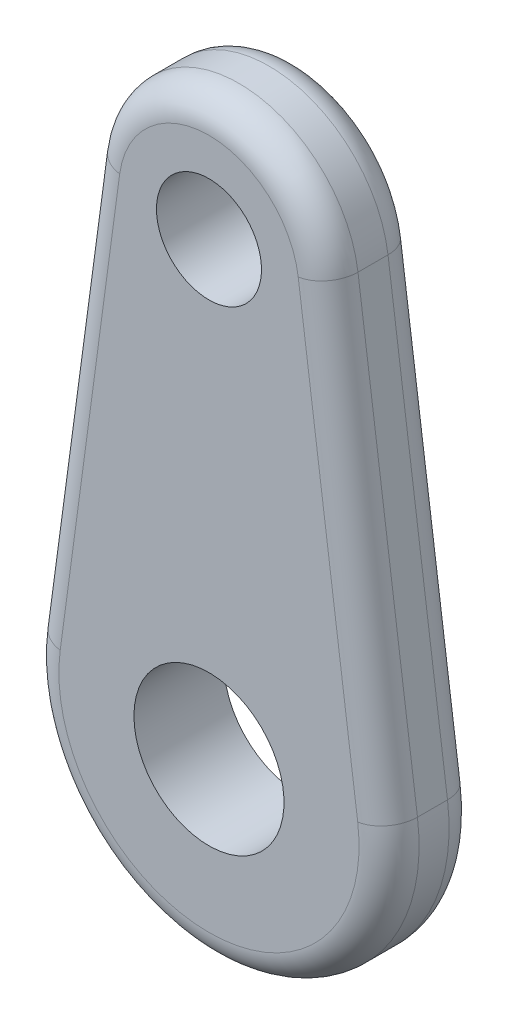
from build123d import *

# Parameters (mm, degrees)
BOSS_EXTRUDE1_DEPTH   = 30
M30_CLEARANCE_HOLE1_D = 35
M45_CLEARANCE_HOLE1_D = 50
FILLET1_R             = 10


with BuildPart() as part:
    # Sketch1 → Boss-Extrude1 (new body)
    with BuildSketch(Plane.XY.offset(30)):
        with BuildLine():
            Line((59.464274989, 8), (39.642849993, 155.333333333))
            ThreePointArc((39.642849993, 155.333333333), (0, 190), (-39.642849993, 155.333333333))
            Line((-39.642849993, 155.333333333), (-59.464274989, 8))
            ThreePointArc((-59.464274989, 8), (0, -60), (59.464274989, 8))
        make_face()
    extrude(amount=-BOSS_EXTRUDE1_DEPTH)

    # M30 Clearance Hole1 (through all)
    with Locations(Plane(origin=(0, 0, 0), x_dir=(-1, 0, 0), z_dir=(0, 0, -1))):
        with Locations((0, 150)):
            Hole(M30_CLEARANCE_HOLE1_D / 2)

    # M45 Clearance Hole1 (through all)
    with Locations(Plane(origin=(0, 0, 0), x_dir=(-1, 0, 0), z_dir=(0, 0, -1))):
        with Locations((0, 0)):
            Hole(M45_CLEARANCE_HOLE1_D / 2)

    # Fillet1
    fillet1_edges = [part.edges().sort_by_distance(p)[0] for p in [
        (0, 190, 0),
        (-49.553562491, 81.666666667, 0),
        (0, -60, 0),
        (-49.553562491, 81.666666667, 30),
        (0, 190, 30),
        (49.553562491, 81.666666667, 30),
        (0, -60, 30),
        (49.553562491, 81.666666667, 0),
    ]]
    fillet(fillet1_edges, radius=FILLET1_R)


solid = part.part
